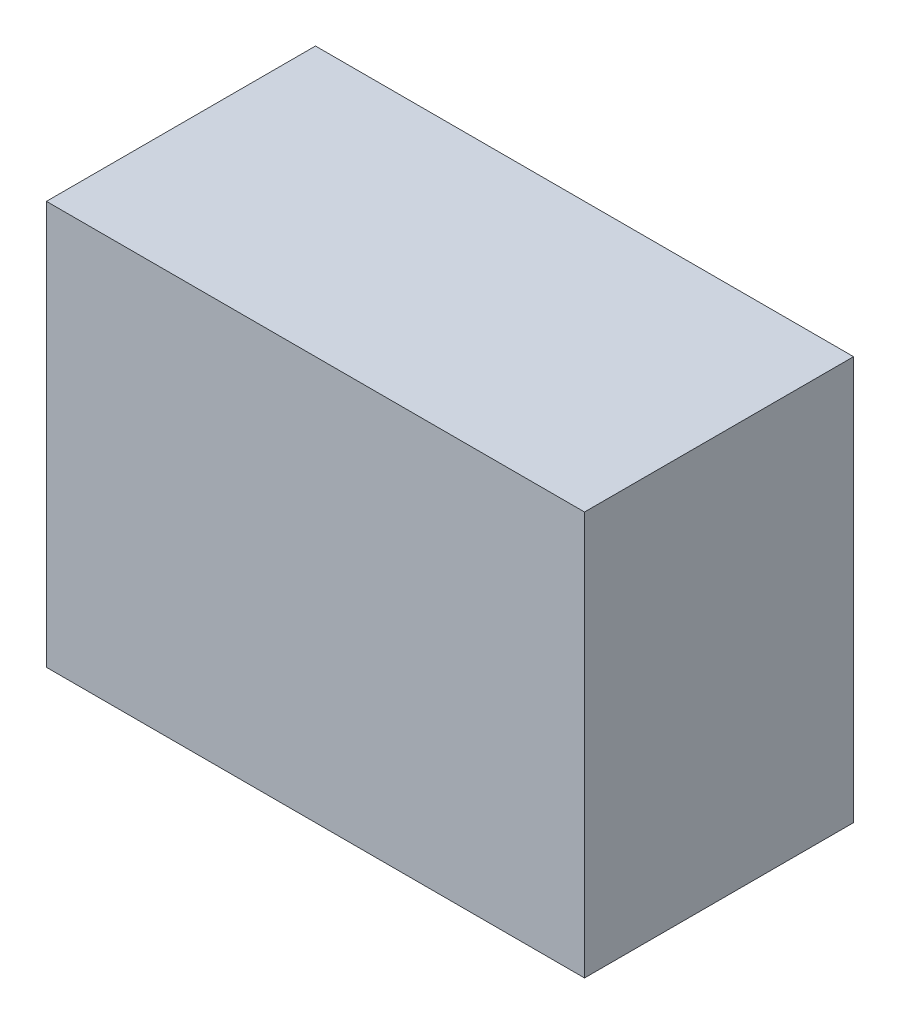
SolidWorks part; units mm, degrees
ref_plane "Front Plane" through (0, 0, 0) normal (0, 0, 1) x (1, 0, 0)
ref_plane "Top Plane" through (0, 0, 0) normal (0, 1, 0) x (1, 0, 0)
ref_plane "Right Plane" through (0, 0, 0) normal (1, 0, 0) x (0, 0, -1)
sketch "Sketch1" plane through (0, 0, 0) normal (0, 1, 0) x (1, 0, 0)
  line L1 (0, 0) -> (20, 0)
  line L2 (0, 0) -> (0, 10)
  line L3 (0, 10) -> (20, 10)
  line L4 (20, 0) -> (20, 10)
  dimension "D1" = 20
  dimension "D2" = 10
extrude "Boss-Extrude1" add sketch "Sketch1" along normal blind 15
